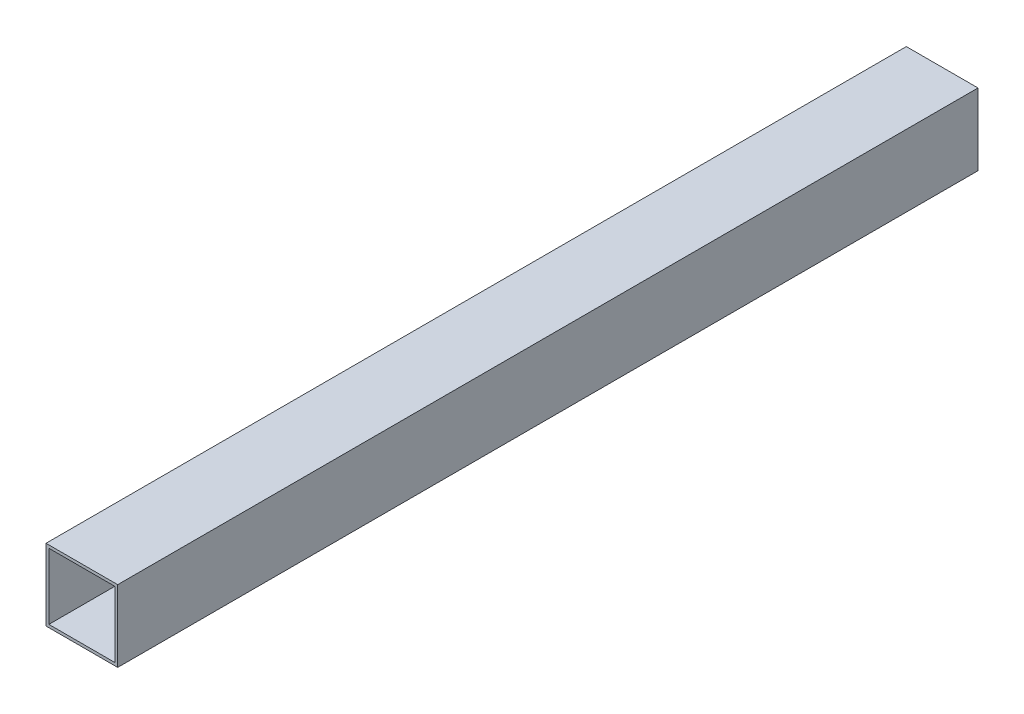
from build123d import *

# Parameters (mm, degrees)
SKETCH1_W           = 50
SKETCH1_H           = 50
SKETCH1_W_2         = 46
SKETCH1_H_2         = 46
BOSS_EXTRUDE1_DEPTH = 600


with BuildPart() as part:
    # Sketch1 → Boss-Extrude1 (new body)
    with BuildSketch(Plane.XY):
        Rectangle(SKETCH1_W, SKETCH1_H)
        Rectangle(SKETCH1_W_2, SKETCH1_H_2, mode=Mode.SUBTRACT)
    extrude(amount=BOSS_EXTRUDE1_DEPTH)


solid = part.part
